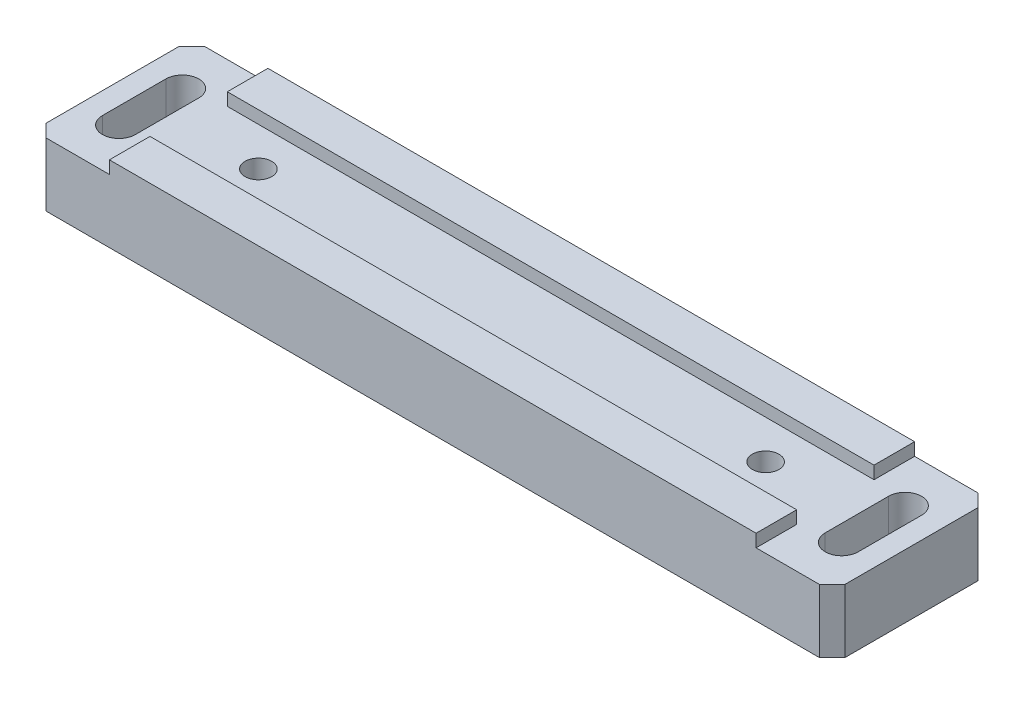
from build123d import *

# Parameters (mm, degrees)
SKETCH_1_W          = 126
SKETCH_1_H          = 25
EXTRUDE_1_DEPTH     = 6
CUT_EXTRUDE_1_DEPTH = 66.339498008
SKETCH_3_W          = 160
SKETCH_3_H          = 12.2
CUT_EXTRUDE_2_DEPTH = 2
CHAMFER_1_SIZE      = 2
HOLE_WIZARD_M5_1_D  = 4.2
SKETCH_8_W          = 42.808580858
SKETCH_8_H          = 66.158715872
SKETCH_8_W_2        = 29.187668767
SKETCH_8_H_2        = 70.606360636
CUT_EXTRUDE_5_DEPTH = 2


with BuildPart() as part:
    # 草图1 → 凸台-拉伸1 (new, symmetric)
    with BuildSketch(Plane(origin=(0, 0, 0), x_dir=(1, 0, 0), z_dir=(0, 1, 0))):
        Rectangle(SKETCH_1_W, SKETCH_1_H)
    extrude(amount=EXTRUDE_1_DEPTH, both=True)

    # 草图2 → 切除-拉伸1 (cut, through all)
    with BuildSketch(Plane(origin=(0, 6, 0), x_dir=(1, 0, 0), z_dir=(0, 1, 0))):
        with BuildLine():
            Line((-54.4, 5), (-54.4, -5))
            ThreePointArc((-54.4, -5), (-57, -7.6), (-59.6, -5))
            Line((-59.6, -5), (-59.6, 5))
            ThreePointArc((-59.6, 5), (-57, 7.6), (-54.4, 5))
        make_face()
    cut_extrude_1 = extrude(amount=-CUT_EXTRUDE_1_DEPTH, mode=Mode.SUBTRACT)

    # 镜向1: 切除-拉伸1 across plane
    add(cut_extrude_1.mirror(Plane(origin=(0, 0, 0), x_dir=(0, 0, 1), z_dir=(1, 0, 0))), mode=Mode.SUBTRACT)

    # 草图3 → 切除-拉伸2 (cut)
    with BuildSketch(Plane(origin=(0, 6, 0), x_dir=(1, 0, 0), z_dir=(0, 1, 0))):
        Rectangle(SKETCH_3_W, SKETCH_3_H)
    extrude(amount=-CUT_EXTRUDE_2_DEPTH, mode=Mode.SUBTRACT)

    # 倒角1
    chamfer_1_edges = [part.edges().sort_by_distance(p)[0] for p in [
        (63, 0, 12.5),
        (-63, 0, 12.5),
        (-63, 0, -12.5),
        (63, 0, -12.5),
    ]]
    chamfer(chamfer_1_edges, length=CHAMFER_1_SIZE)

    # M5 螺纹孔1 (through all)
    with Locations(Plane(origin=(0, 4, 0), x_dir=(1, 0, 0), z_dir=(0, 1, 0))):
        with Locations((-40, 0), (40, 0)):
            Hole(HOLE_WIZARD_M5_1_D / 2)

    # 草图8 → 切除-拉伸5 (cut)
    with BuildSketch(Plane(origin=(0, 6, 0), x_dir=(1, 0, 0), z_dir=(0, 1, 0))):
        with Locations((-72.404290429, 14.176867687)):
            Rectangle(SKETCH_8_W, SKETCH_8_H)
        with Locations((65.593834383, 18.207545755)):
            Rectangle(SKETCH_8_W_2, SKETCH_8_H_2)
    extrude(amount=-CUT_EXTRUDE_5_DEPTH, mode=Mode.SUBTRACT)


solid = part.part
